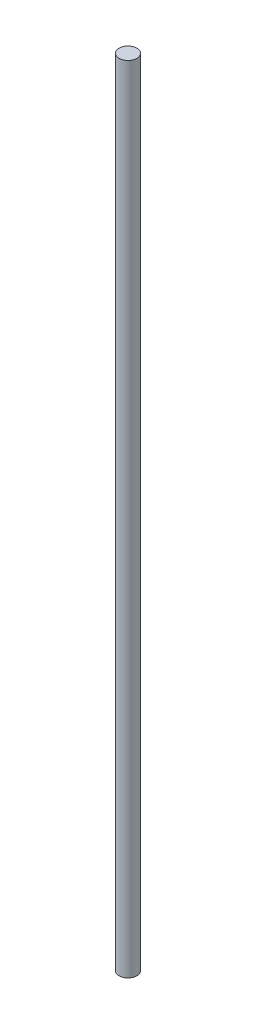
SolidWorks part; units mm, degrees
ref_plane "Front Plane" through (0, 0, 0) normal (0, 0, 1) x (1, 0, 0)
ref_plane "Top Plane" through (0, 0, 0) normal (0, 1, 0) x (1, 0, 0)
ref_plane "Right Plane" through (0, 0, 0) normal (1, 0, 0) x (0, 0, -1)
sketch "Sketch1" plane through (0, 0, 0) normal (0, 1, 0) x (1, 0, 0)
  circle A0 centre (0, 0) radius 125
  dimension "D1" = 250
extrude "Boss-Extrude1" add sketch "Sketch1" along normal blind 11200
